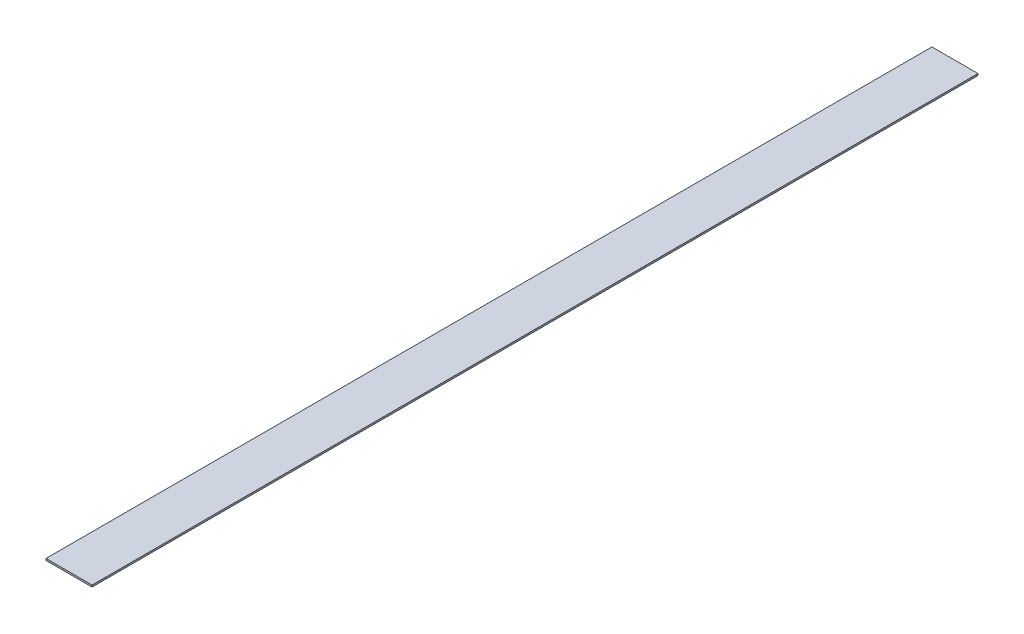
from build123d import *

# Parameters (mm, degrees)
SKETCH1_W           = 260
SKETCH1_H           = 10
BOSS_EXTRUDE1_DEPTH = 5000


with BuildPart() as part:
    # Sketch1 → Boss-Extrude1 (new body)
    with BuildSketch(Plane.XY):
        with Locations((130, 5)):
            Rectangle(SKETCH1_W, SKETCH1_H)
    extrude(amount=BOSS_EXTRUDE1_DEPTH)


solid = part.part
